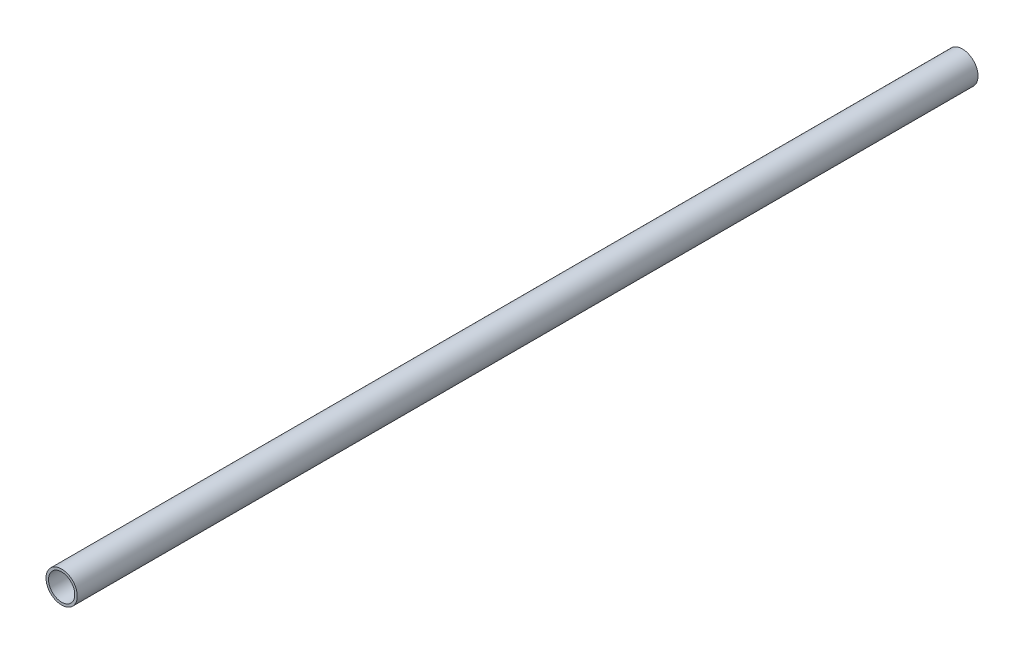
from build123d import *

# Parameters (mm, degrees)
SKETCH_1_R      = 12.5
SKETCH_1_R_2    = 10.5
EXTRUDE_1_DEPTH = 360


with BuildPart() as part:
    # 草图1 → 凸台-拉伸1 (new, symmetric)
    with BuildSketch(Plane.XY):
        with Locations(Location((0, 0, 0), (0, 0, 180))):
            Circle(SKETCH_1_R)
        with Locations(Location((0, 0, 0), (0, 0, 180))):
            Circle(SKETCH_1_R_2, mode=Mode.SUBTRACT)
    extrude(amount=EXTRUDE_1_DEPTH, both=True)


solid = part.part
